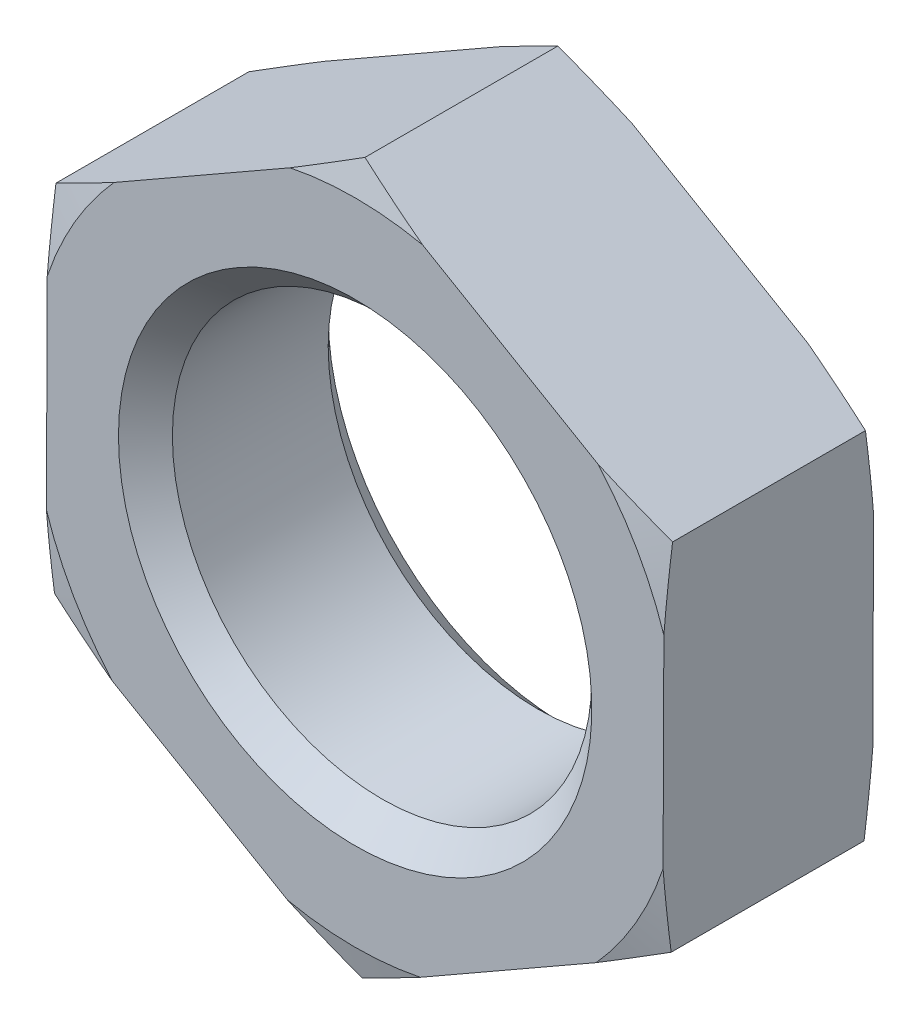
SolidWorks part; units mm, degrees
extrude "Base-Extrude" add sketch "Sketch1" along normal blind 21
sketch "Sketch1" plane through (0, 0, 0) normal (0, 0, 1) x (1, 0, 0)
  line L0 (-26.8088, 0) -> (37.1748, 0) construction
  line L1 (0, 25.0215) -> (0, -25.0215) construction
  line L3 (0.1402, 35.6497) -> (-30.8034, 17.9463)
  line L4 (-30.8034, 17.9463) -> (-30.9437, -17.7034)
  line L5 (-30.9437, -17.7034) -> (-0.1402, -35.6497)
  line L6 (-0.1402, -35.6497) -> (30.8034, -17.9463)
  line L7 (30.8034, -17.9463) -> (30.9437, 17.7034)
  line L8 (30.9437, 17.7034) -> (0.1402, 35.6497)
  circle A0 centre (0, 0) radius 30.8738 construction
  circle A1 centre (0, 0) radius 21
cosmetic thread "Cosmetic Thread1"
chamfer "Chamfer1" distance 2.7 angle 45 2 edges at (21, 0, 0) (21, 0, 21)
material "04级"
ref_plane "Plane1" through (0, 0, 0) normal (0, 0, 1) x (1, 0, 0)
ref_plane "Plane2" through (0, 0, 0) normal (0, 1, 0) x (1, 0, 0)
ref_plane "Plane3" through (0, 0, 0) normal (1, 0, 0) x (0, 0, -1)
sketch "Dimension Sketch" plane through (0, 0, 0) normal (0, 0, 1) x (1, 0, 0)
  line L0 (0, 0) -> (24.1005, 0)
  line L1 (27.4249, 65.7219) -> (72.8249, 65.7219)
  line L2 (46.8781, 65.7219) -> (106.8781, 65.7219)
  line L3 (-37.8187, 0) -> (2.1813, 0)
  point P3 (42, 0)
  point P4 (1.5, 0)
  point P5 (71.3, 0)
  point P6 (21, 0)
  point P7 (24.32, 0)
  point P8 (65, 0)
sketch "Sketch2" plane through (0, 0, 0) normal (0, 0, -1) x (-1, 0, 0)
  circle A0 centre (0, 0) radius 32.5
  circle A1 centre (0, 0) radius 21 construction
extrude "Cut-Extrude1" cut sketch "Sketch2" against normal through all draft 75 flip side to cut
sketch "Sketch3" plane through (0, 0, 21) normal (0, 0, 1) x (1, 0, 0)
  circle A0 centre (0, 0) radius 32.5
extrude "Cut-Extrude2" cut sketch "Sketch3" against normal through all draft 75 flip side to cut
equation "\"e@Sketch1\" = \"e@Dimension Sketch\""
equation "\"D1@Dimension Sketch\" = \"D@Dimension Sketch\" / 1.05"
equation "\"D@Sketch1\" = \"D@Dimension Sketch\""
equation "\"m@Base-Extrude\" = \"m@Dimension Sketch\""
equation "\"D1@Sketch3\" = \"s@Dimension Sketch\""
equation "\"s@Sketch2\" = \"s@Dimension Sketch\""
equation "\"D2@Cosmetic Thread1\" = 1.05 * \"D1@Dimension Sketch\""
equation "\"D1@Chamfer1\" =  ( \"da@Dimension Sketch\" - \"D1@Dimension Sketch\" )  / 2"
